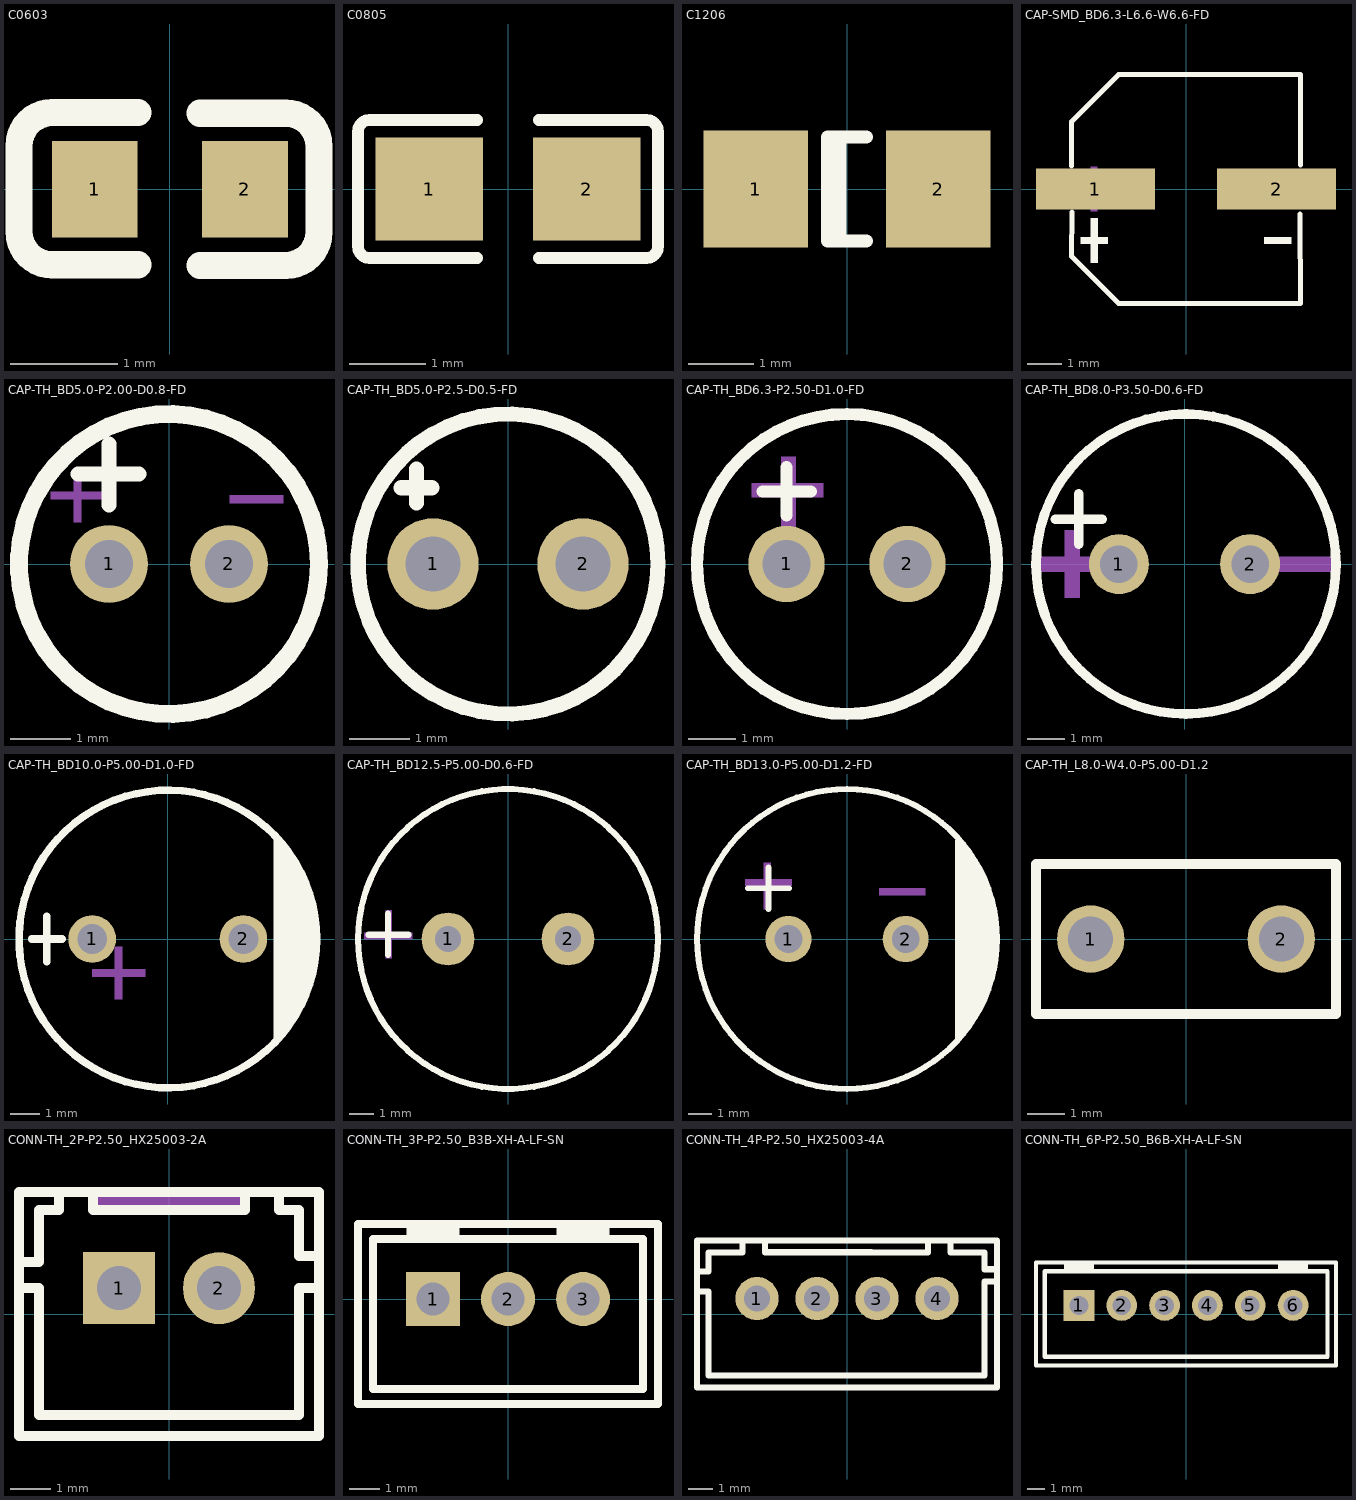
[diagram p0: the footprints below, top view; thin cyan lines are the x and y axes]
# Altium footprint library MISC84402-3.PcbLib: 74 footprints (part 1 of 5)
Each footprint in its own frame and in the unit in brackets; x right, y up, seen from the top. Pads: shape width x height; smd on the part's side, far side on the other; paste and mask are expansions set on the pad; w line width, h text height; cw(c..) or ccw(c..) is an arc to the next point about the centre after c.

## C0603 [mm]
pads (2):
  rect 0.8x0.9 smd: 1(-0.7,0) 2(0.7,0)
Top Overlay:
  lines w0.254: -0.296,-0.704 -1.096,-0.704 cw(c-1.096,-0.394) -1.406,-0.394 -1.405,0.406 cw(c-1.096,0.406) -1.096,0.715 -0.296,0.715 ; 0.28,-0.71 1.08,-0.71 ccw(c1.08,-0.4) 1.39,-0.4 1.39,0.4 ccw(c1.08,0.4) 1.08,0.71 0.28,0.71

## C0805 [mm]
pads (2):
  rect 1.41x1.35 smd: 1(-1.03,0) 2(1.03,0)
Top Overlay:
  lines w0.152: -0.401,-0.904 -1.811,-0.904 cw(c-1.811,-0.751) -1.964,-0.751 -1.964,0.751 cw(c-1.811,0.751) -1.811,0.904 -0.401,0.904 ; 0.401,-0.904 1.811,-0.904 ccw(c1.811,-0.751) 1.964,-0.751 1.964,0.751 ccw(c1.811,0.751) 1.811,0.904 0.401,0.904
Top Paste:
  region: -1.675,-0.62 -1.675,0.66 -1.625,0.71 -0.475,0.71 -0.425,0.66 -0.42,0.25 -0.87,0.25 -0.87,-0.2 -0.43,-0.2 -0.425,-0.62 -0.475,-0.67 -1.625,-0.67
  region: 0.475,-0.62 0.475,-0.2 0.92,-0.2 0.92,0.25 0.48,0.25 0.475,0.66 0.525,0.71 1.675,0.71 1.725,0.66 1.725,-0.62 1.675,-0.67 0.525,-0.67

## C1206 [mm] "Chip Capacitor; Body 3.2 x 1.6 mm (LxW typ)"
height 1.35
pads (2):
  rect 1.6x1.8 smd: 1(-1.4,0) 2(1.4,0)
Top Overlay:
  lines w0.2: -0.11,-0.8 -0.11,0.8 ; 0.3,-0.8 -0.3,-0.8 -0.3,0.8 0.3,0.8

## CAP-SMD_BD6.3-L6.6-W6.6-FD [mm]
pads (2):
  rect 3.5x1.2 smd: 1(-2.67,0) 2(2.67,0)
Top Overlay:
  region: 3.102,-1.419 3.102,-1.617 2.31,-1.617 2.31,-1.419
  region: -3.102,-1.419 -3.102,-1.617 -2.31,-1.617 -2.31,-1.419
  region: -2.805,-0.858 -2.805,-2.178 -2.607,-2.178 -2.607,-0.858
  lines w0.152: -3.376,0.686 -3.376,1.98 -1.98,3.376 3.376,3.376 3.369,0.707 ; -3.362,-0.686 -3.376,-1.981 -1.981,-3.376 3.376,-3.376 3.356,-0.74
Mechanical 15:
  region: 3.102,0.099 3.102,-0.099 2.31,-0.099 2.31,0.099
  region: -3.102,0.099 -3.102,-0.099 -2.31,-0.099 -2.31,0.099
  region: -2.81,0.66 -2.81,-0.66 -2.612,-0.66 -2.612,0.66

## CAP-TH_BD5.0-P2.00-D0.8-FD [mm]
pads (2):
  round 1.3 hole 0.8: 1(-1,0) 2(1,0)
Top Overlay:
  circle w0.3: c0,0 r2.5
  lines w0.254: -1.516,1.5 -0.5,1.5 ; -1,0.984 -1,2
Mechanical 15:
  region: 1.016,1.143 1.905,1.143 1.905,1.016 1.016,1.016
  region: -1.588,0.699 -1.588,1.587 -1.461,1.587 -1.46,0.699
  region: -1.969,1.206 -1.08,1.206 -1.08,1.079 -1.969,1.079

## CAP-TH_BD5.0-P2.5-D0.5-FD [mil]
pads (2):
  round 60 hole 36: 1(-49.21,0) 2(49.21,0)
Top Overlay:
  circle w10: c0,0 r98.43
  lines w10: -70,50 -50,50 ; -60,40 -60,62.4

## CAP-TH_BD6.3-P2.50-D1.0-FD [mm]
pads (2):
  round 1.6 hole 1: 1(-1.27,0) 2(1.27,0)
Top Overlay:
  circle w0.254: c0,0 r3.15
  lines w0.254: -1.778,1.524 -0.762,1.524 ; -1.27,1.016 -1.27,2.032
Mechanical 15:
  region: -2,1.7 -0.5,1.7 -0.5,1.4 -2,1.4
  region: -1.381,0.752 -1.381,2.252 -1.081,2.252 -1.081,0.752

## CAP-TH_BD8.0-P3.50-D0.6-FD [mm]
pads (2):
  round 1.6 hole 1: 1(-1.75,0) 2(1.75,0)
Top Overlay:
  lines w0.254: -3.445,1.2 -2.2,1.2 ; -2.822,0.527 -2.822,1.873 ; 0.003,4 ccw(c0.038,0.001) 0.074,4
Mechanical 15:
  region: 2.1,0.2 2.1,-0.2 3.9,-0.2 3.9,0.2
  region: -3.9,0.2 -3.9,-0.2 -2.1,-0.2 -2.1,0.2
  region: -3.2,-0.9 -2.8,-0.9 -2.8,0.9 -3.2,0.9

## CAP-TH_BD10.0-P5.00-D1.0-FD [mm]
pads (2):
  round 1.6 hole 1: 1(-2.54,0) 2(2.54,0)
Top Overlay:
  circle w0.254: c0,0 r5
  region: 3.556,3.556 3.556,-3.556 4.318,-2.54 4.826,-1.016 5.08,0.508 4.826,1.524
  lines w0.254: -4.572,0 -3.556,0 ; -4.064,-0.762 -4.064,0.762
Mechanical 15:
  region: -1.778,-2.032 -1.524,-2.032 -1.524,-0.254 -1.778,-0.254
  region: -2.54,-1.016 -0.762,-1.016 -0.762,-1.27 -2.54,-1.27

## CAP-TH_BD12.5-P5.00-D0.6-FD [mm]
pads (2):
  round 2.2 hole 1.1: 1(-2.5,0) 2(2.5,0)
Top Overlay:
  circle w0.254: c0,0 r6.25
  lines w0.254: -5.817,0.178 -4.14,0.178 ; -5.004,-0.66 -5.004,1.067
Mechanical 15:
  region: -6,0.25 -4,0.25 -4,0 -6,0
  region: -5.092,-0.811 -5.092,1.189 -4.842,1.189 -4.842,-0.811

## CAP-TH_BD13.0-P5.00-D1.2-FD [mm]
pads (2):
  round 2 hole 1.2: 1(-2.539,0) 2(2.541,0)
Top Overlay:
  circle w0.254: c0,0 r6.5
  region: 4.701,4.3 4.701,-4.5 5.801,-3 6.301,-1.7 6.401,-0.5 6.301,1.5 5.701,3.2
  lines w0.254: -4.3,2.2 -2.5,2.2 ; -3.4,1.3 -3.4,3.1
Mechanical 15:
  region: 1.401,2.2 3.401,2.2 3.401,1.9 1.401,1.9
  region: -3.599,1.3 -3.599,3.3 -3.499,3.3 -3.299,3.3 -3.299,1.3
  region: -4.399,2.6 -2.399,2.6 -2.399,2.3 -4.399,2.3
  region: 4.722,4.286 4.722,-4.514 5.822,-3.014 6.322,-1.714 6.422,-0.514 6.322,1.486 5.722,3.186

## CAP-TH_L8.0-W4.0-P5.00-D1.2 [mm]
pads (2):
  round 1.8 hole 1.2: 1(-2.54,0) 2(2.54,0)
Top Overlay:
  lines w0.254: -4,-2 -4,2 4,2 4,-2 -4,-2

## CONN-TH_2P-P2.50_HX25003-2A [mm]
pads (2):
  rect 1.8x1.8 hole 1.1: 1(-1.25,0.646)
  round 1.8 hole 1.1: 2(1.25,0.646)
Top Overlay:
  lines w0.254: -3.75,-1.769 -3.75,0.646 -3.25,0.646 -3.25,-1.769 -3.25,-2.521 3.25,-2.521 3.25,-1.698 3.25,0.646 3.75,0.646 3.75,-1.698 ; -3.75,-0.957 -3.75,1.294 -3.25,1.296 -3.25,2.604 -2.75,2.604 -2.75,3.054 ; -1.9,2.596 -1.9,3.046 ; -1.9,2.604 1.9,2.604 ; 1.9,2.596 1.9,3.046 ; 2.75,2.596 2.75,3.045 ; 2.75,2.604 3.25,2.604 3.25,1.446 3.75,1.446 3.75,-0.855 ; -3.75,-3.054 3.75,-3.054 3.75,3.046 -3.75,3.046 -3.75,-3.054
Mechanical 15:
  region: 1.9,3.046 1.9,2.546 -1.9,2.546 -1.9,3.046

## CONN-TH_3P-P2.50_B3B-XH-A-LF-SN [mm]
pads (3):
  rect 1.8x1.8 hole 1.1: 1(-2.5,0)
  round 1.8 hole 1.1: 2(0,0) 3(2.5,0)
Top Overlay:
  lines w0.254: -3.251,1.999 -3.251,2.499 ; -3.251,2.25 -1.749,2.25 ; -1.749,1.999 -1.749,2.499 ; 1.75,2.001 1.75,2.501 ; 1.75,2.251 3.25,2.251 ; 3.25,2.001 3.25,2.501 ; -5,-3.499 4.999,-3.499 4.999,2.5 -5,2.5 -5,-3.499 ; -4.5,-2.999 4.5,-2.999 4.5,2 -4.5,2 -4.5,-2.999

## CONN-TH_4P-P2.50_HX25003-4A [mm]
pads (4):
  round 1.8 hole 1.1: 1(-3.75,0.645) 2(-1.25,0.645) 3(1.25,0.645) 4(3.75,0.645)
Top Overlay:
  lines w0.254: -6.25,-3.055 -6.25,3.045 ; -6.25,-3.055 6.25,-3.055 ; -6.25,1.775 -5.775,1.775 -5.775,2.57 -4.361,2.57 -4.361,3.02 ; -6.25,3.055 6.24,3.055 ; -6.24,0.945 -5.775,0.945 -5.775,-2.555 5.726,-2.555 5.726,1.356 6.226,1.356 ; -3.424,3.021 -3.424,2.571 1.019,2.571 0.976,2.57 ; 1.019,2.57 3.375,2.57 3.375,3.02 ; 4.31,2.571 4.31,3.019 ; 4.314,2.57 5.726,2.57 5.726,1.864 6.226,1.864 ; 6.25,-3.055 6.25,3.045

## CONN-TH_6P-P2.50_B6B-XH-A-LF-SN [mm]
pads (6):
  rect 1.8x1.8 hole 1.1: 1(-6.251,0.501)
  round 1.8 hole 1.1: 2(-3.749,0.499) 3(-1.249,0.499) 4(1.251,0.499) 5(3.751,0.499) 6(6.251,0.499)
Top Overlay:
  lines w0.254: -7,2.5 -7,3 ; -7,2.75 -5.5,2.75 ; -5.5,2.5 -5.5,3 ; 5.501,2.5 5.501,3 ; 5.501,2.75 7.001,2.75 ; 7.001,2.5 7.001,3 ; -8.75,-3 -8.75,3 8.75,3 8.75,-3 -8.75,-3 ; -8.25,-2.5 -8.25,2.5 8.251,2.5 8.251,-2.5 -8.25,-2.5